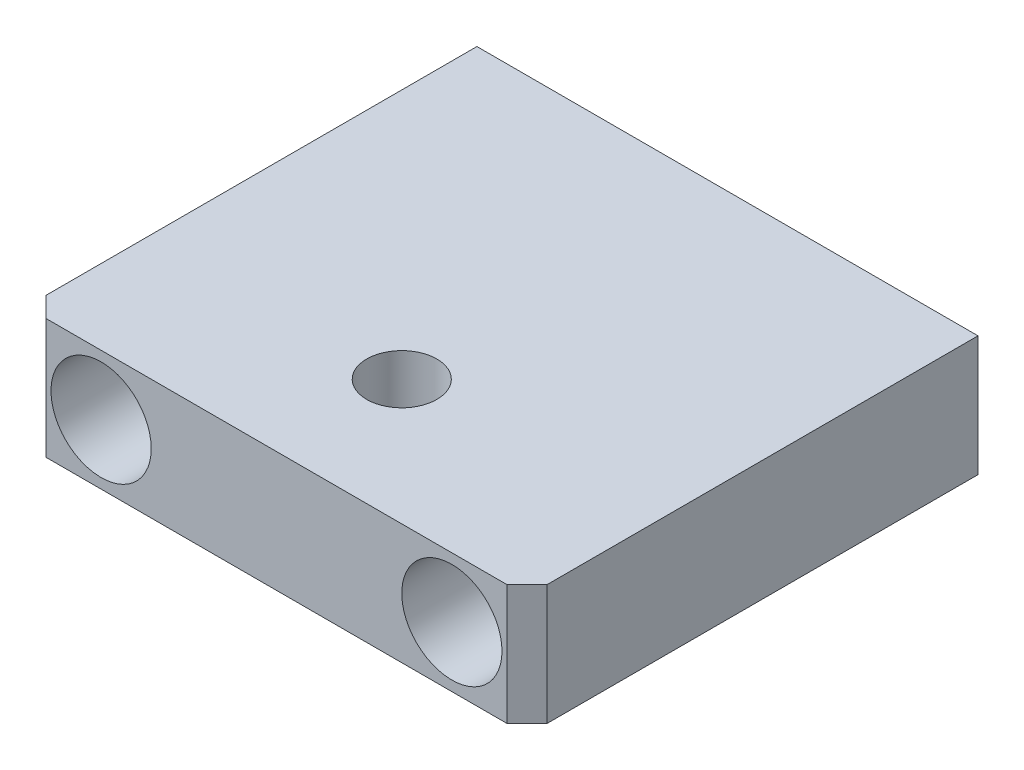
SolidWorks part; units mm, degrees
material "A5052"
ref_plane "Front Plane" through (0, 0, 0) normal (0, 0, 1) x (1, 0, 0)
ref_plane "Top Plane" through (0, 0, 0) normal (0, 1, 0) x (1, 0, 0)
ref_plane "Right Plane" through (0, 0, 0) normal (1, 0, 0) x (0, 0, -1)
sketch "Sketch1" plane through (0, 0, 0) normal (0, 0, 1) x (1, 0, 0)
  line L1 (25, -6) -> (-25, -6)
  line L2 (25, -6) -> (25, 6)
  line L3 (25, 6) -> (-25, 6)
  line L4 (-25, -6) -> (-25, 6)
  line L5 (25, -6) -> (-25, 6) construction
  line L6 (25, 6) -> (-25, -6) construction
  point P0 (0, 0)
  dimension "D1" = 12
  dimension "D2" = 50
extrude "Boss-Extrude1" add sketch "Sketch1" along normal mid plane 45
hole_wizard "M8x1.0 Tapped Hole1" positions "Sketch3" profile "Sketch2" tap size "M8x1.0" standard "GB" end condition up to next
sketch "Sketch3" plane through (0, 6, 0) normal (0, 1, 0) x (1, 0, 0)
  line L3 (0, 0) -> (-26.3179, 0) construction
  point P8 (0, -10)
sketch "Sketch2" plane through (0, 6, 10) normal (1, 0, 0) x (0, 0, 1)
  line L0 (0, 0) -> (0, 12)
  line L1 (0, 12) -> (3.5, 12)
  line L2 (3.5, 12) -> (3.5, 0)
  line L5 (3.5, 0) -> (0, 0)
  line L11 (0, -6.35) -> (0, 107.95) construction
  dimension "通孔螺纹孔钻头直径" = 7
  dimension "通孔螺纹孔钻头深度" = 12
cosmetic thread "Hole thread 1"
hole_wizard "Hex socket cap screw hole type 1" positions "Sketch5" profile "Sketch4" counterbore size "M5" standard "GB" end condition up to next
sketch "Sketch5" plane through (0, 0, 22.5) normal (0, 0, 1) x (1, 0, 0)
  line L0 (0, 13.7803) -> (0, 0) construction
  line L1 (0, 0) -> (-26.9965, 0) construction
  point P0 (-17.5, 0)
  point P10 (17.5, 0)
  dimension "D1" = 17.5
sketch "Sketch4" plane through (-17.5, 0, 22.5) normal (1, 0, 0) x (0, -1, 0)
  line L0 (0, 0) -> (0, 45)
  line L1 (0, 45) -> (2.75, 45)
  line L3 (2.75, 45) -> (2.75, 35)
  line L4 (2.75, 35) -> (5, 35)
  line L5 (5, 35) -> (5, 0)
  line L7 (5, 0) -> (0, 0)
  line L11 (0, -6.35) -> (0, 107.95) construction
  dimension "通孔孔直径" = 5.5
  dimension "通孔孔深度" = 45
  dimension "柱形沉头孔直径" = 10
  dimension "柱形沉头孔深度" = 35
chamfer "Chamfer1" distance 2 angle 45 2 edges at (-25, 0, 22.5) (25, 0, 22.5)
